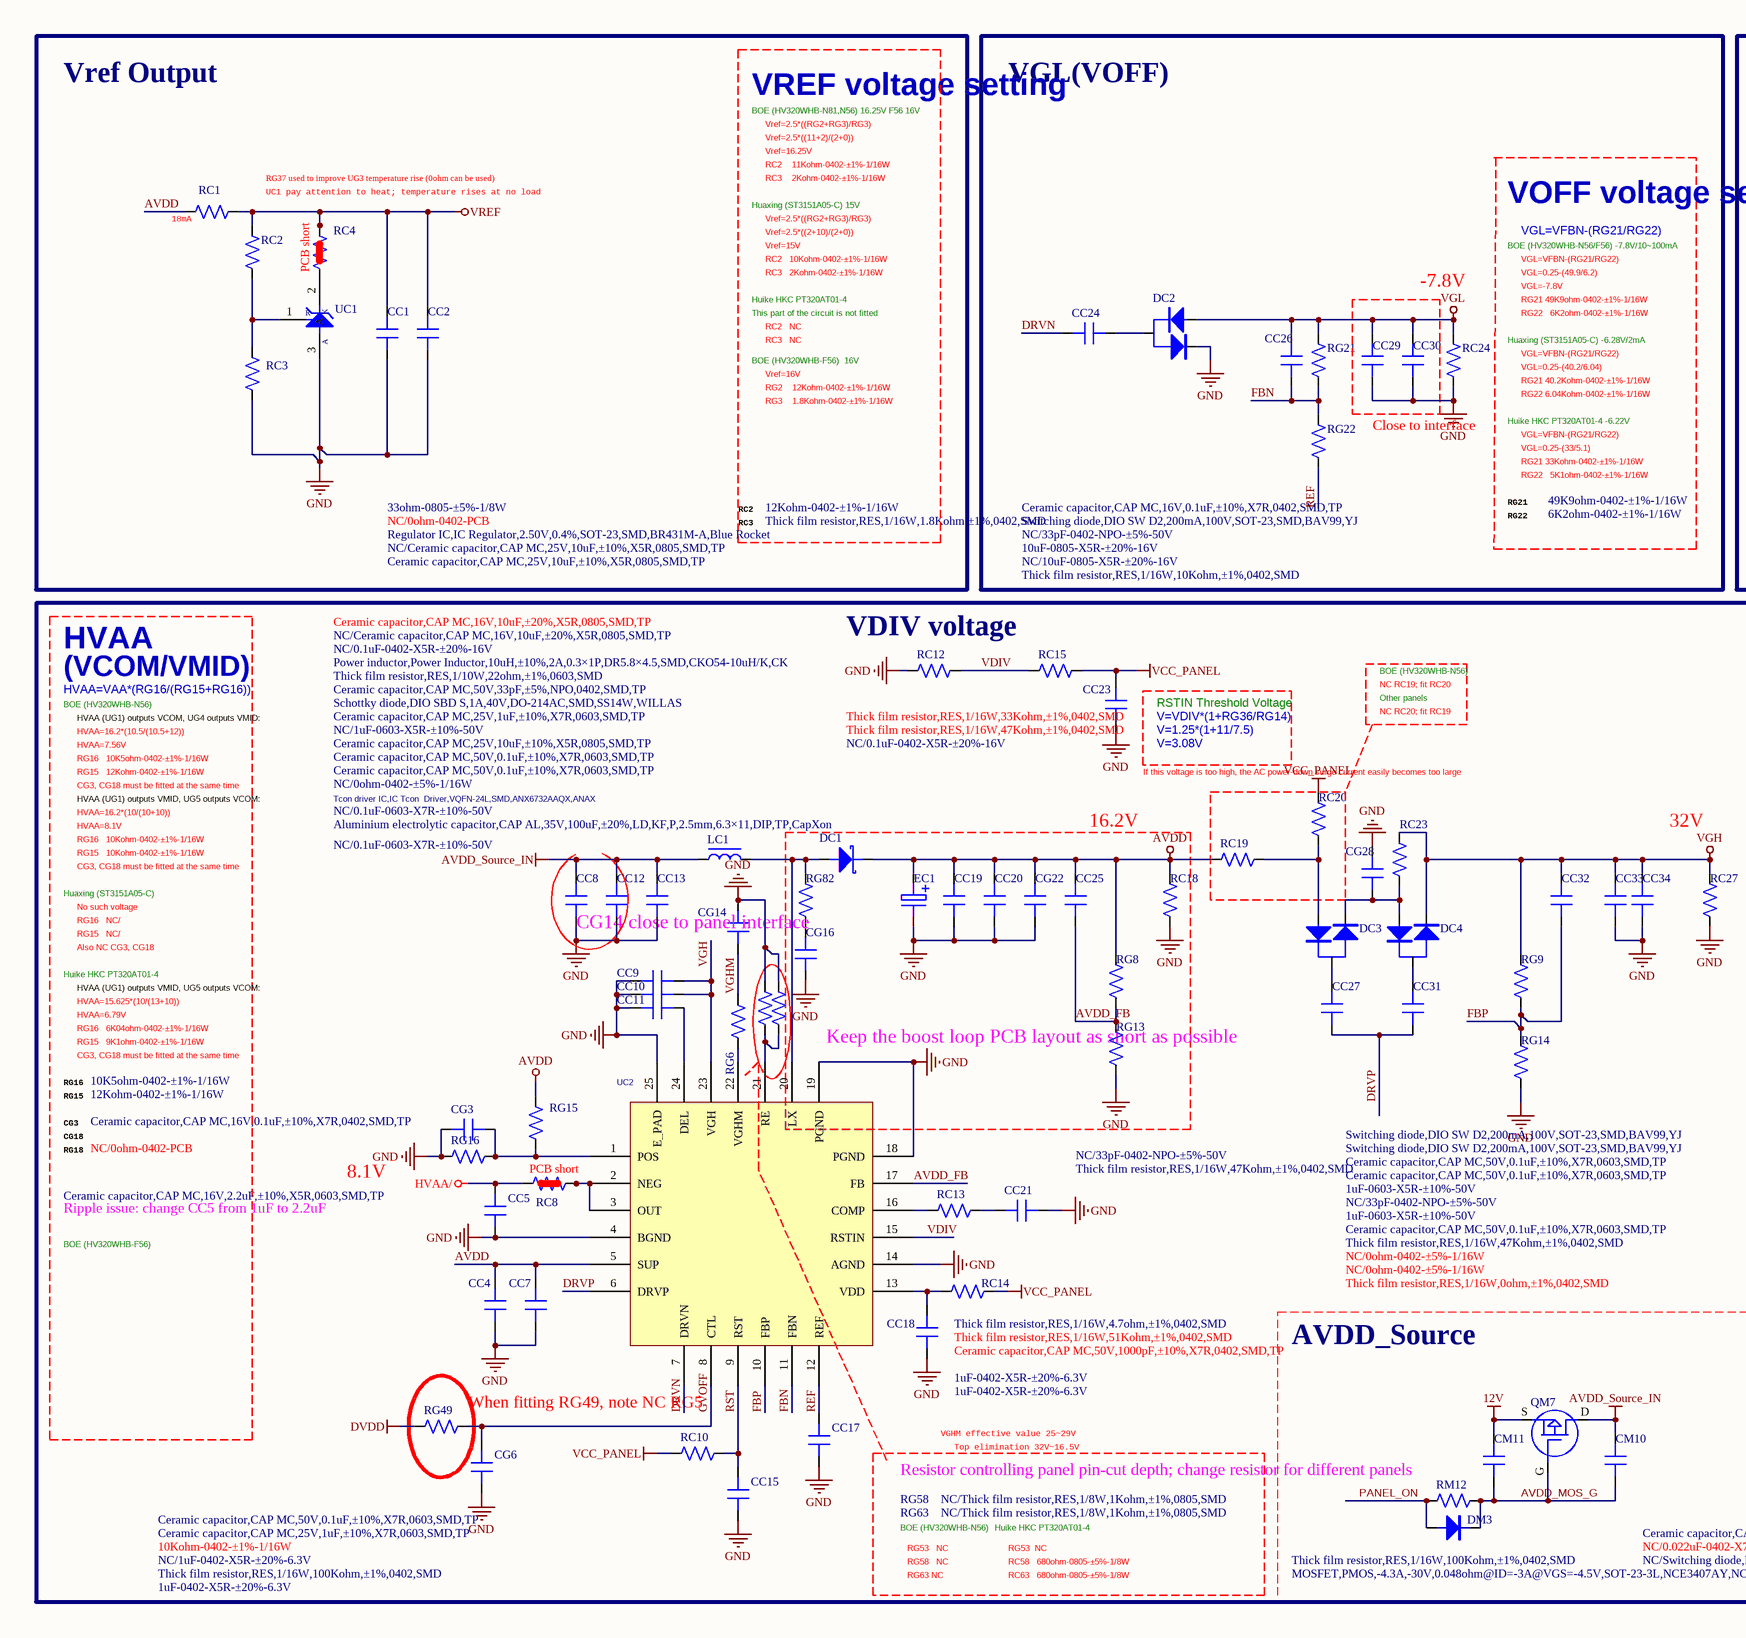
[diagram p0: MISC86383-19.SchDoc, left]
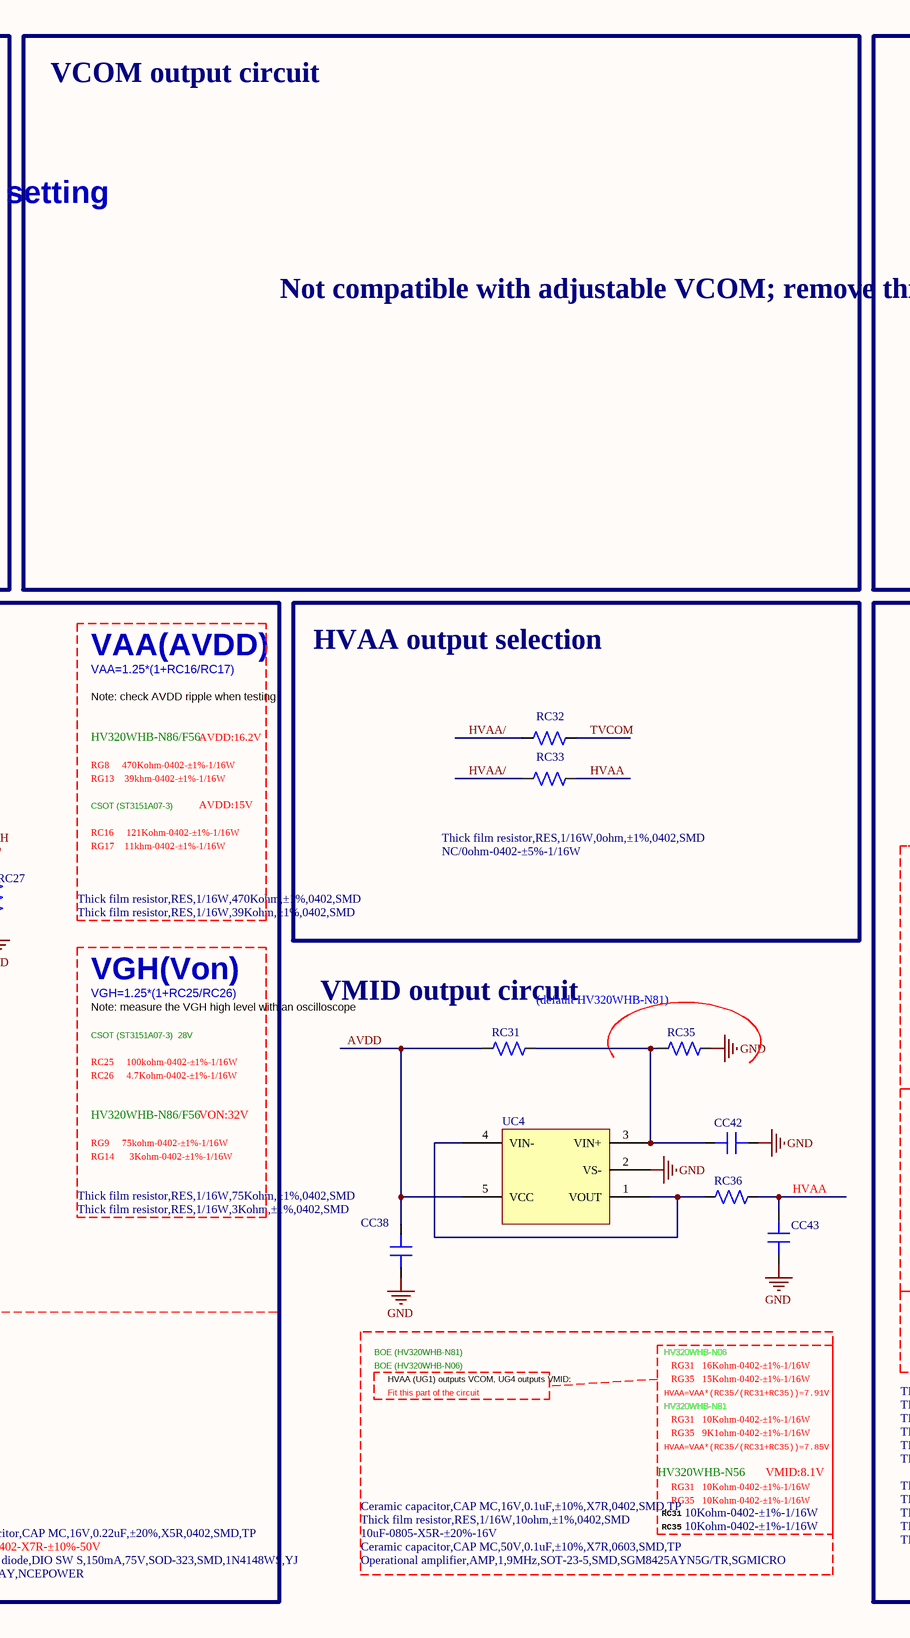
[diagram p1: MISC86383-19.SchDoc, middle]
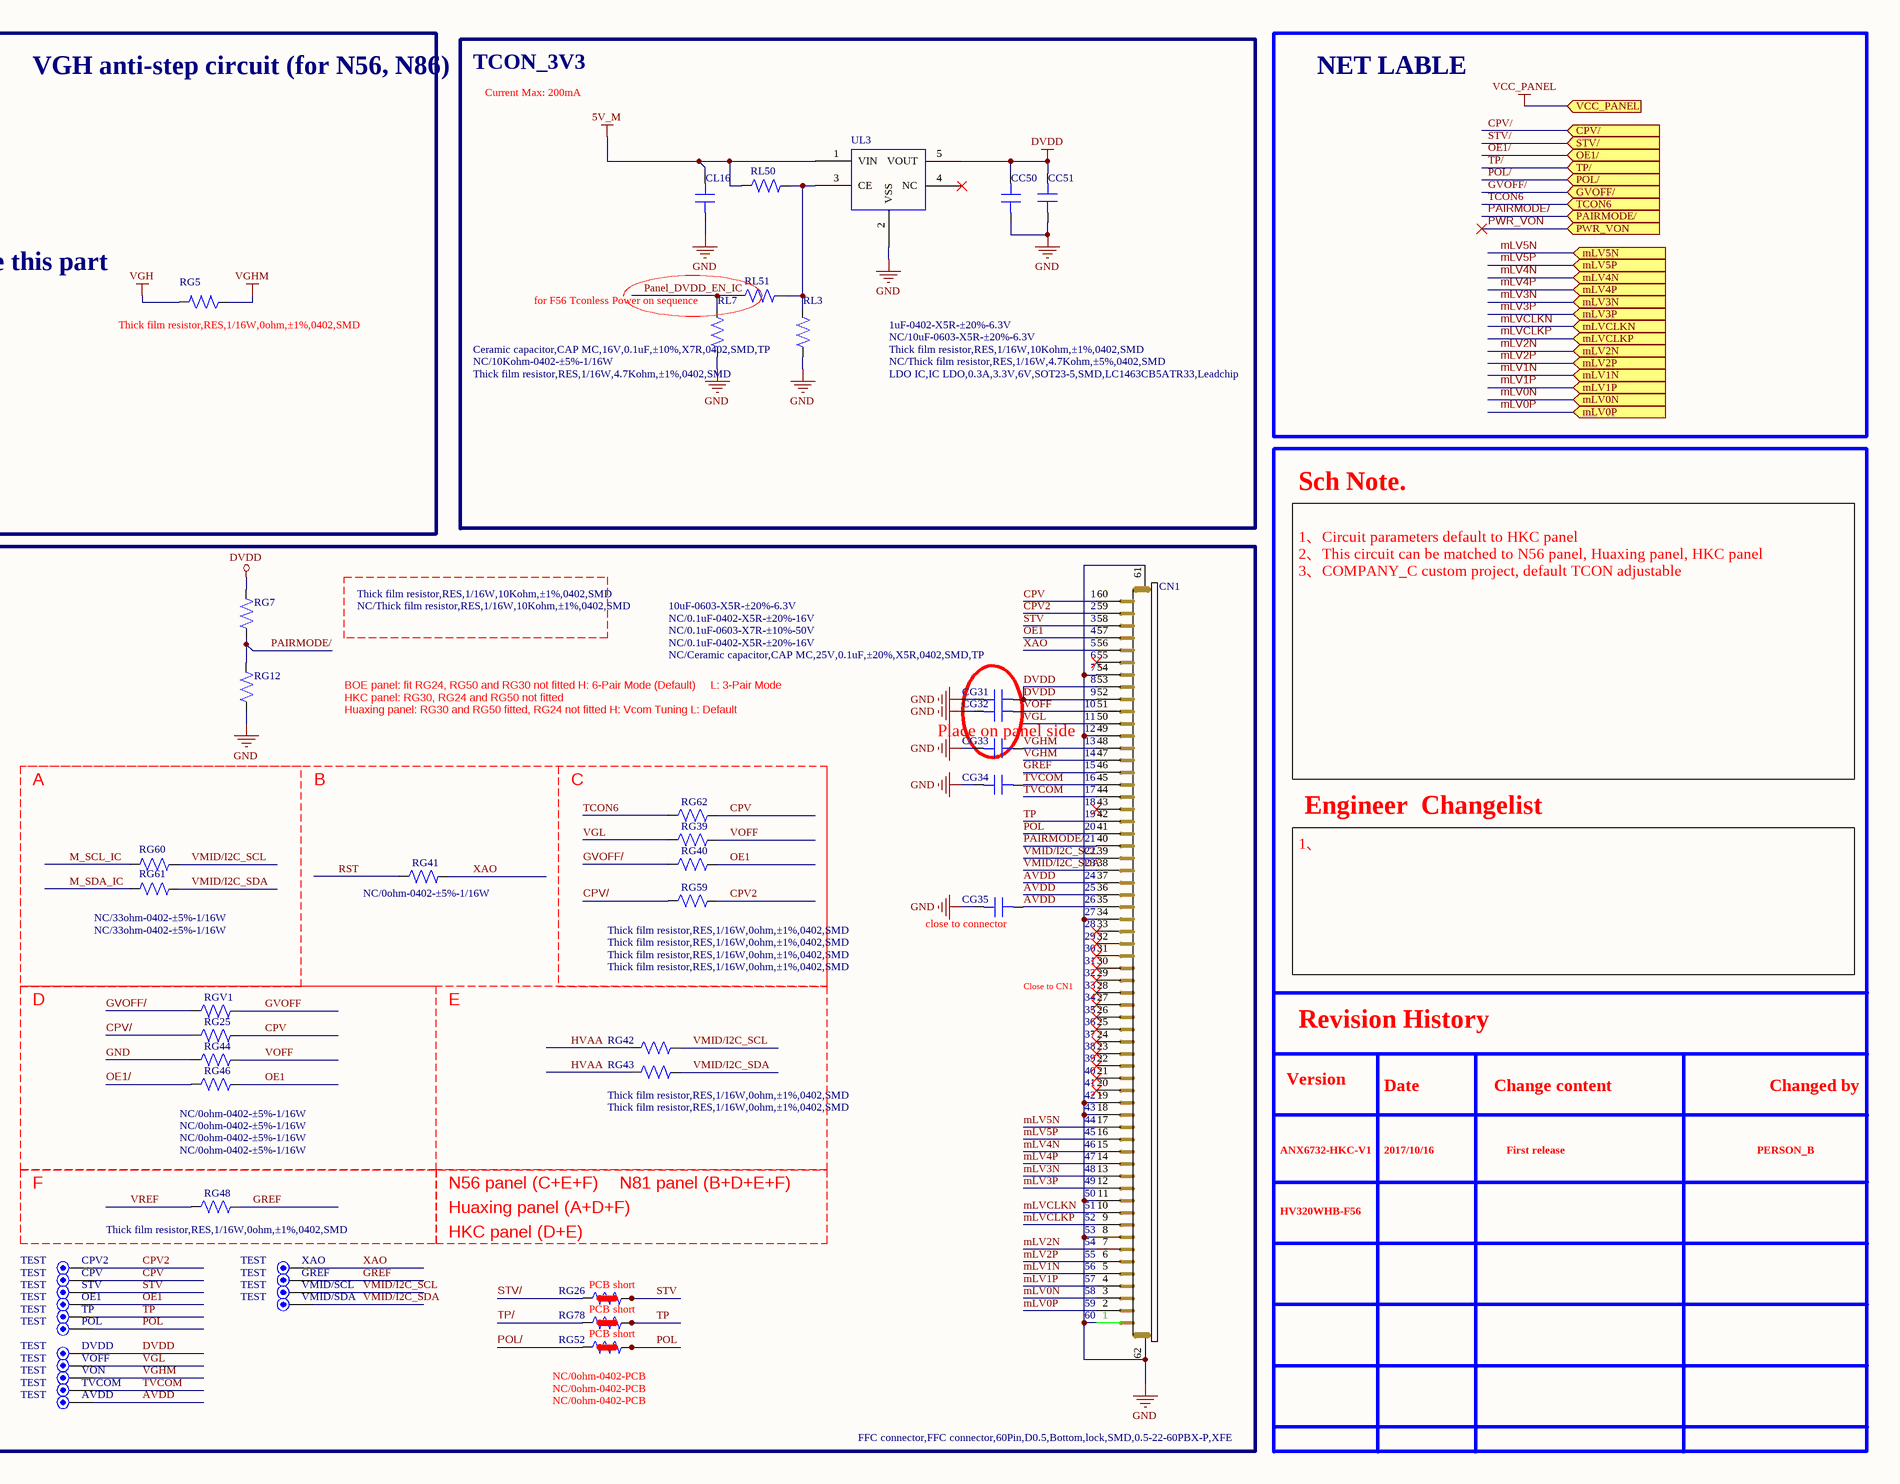
[diagram p2: MISC86383-19.SchDoc, right]
# Altium project MISC86383-33.PrjPCB (part 6 of 8)

## Sheet MISC86383-19.SchDoc
size 914 x 330 mm

### Parts
AVDD  TEST  [TP]
CC1  NC/Ceramic capacitor,CAP MC,25V,10uF,±10%,X5R,0805,SMD,TP  [C0805]
CC2  Ceramic capacitor,CAP MC,25V,10uF,±10%,X5R,0805,SMD,TP  [C0805]
CC4  Ceramic capacitor,CAP MC,25V,1uF,±10%,X7R,0603,SMD,TP  [C0603]
CC5  Ceramic capacitor,CAP MC,16V,2.2uF,±10%,X5R,0603,SMD,TP  [C0603]
CC7  Ceramic capacitor,CAP MC,50V,0.1uF,±10%,X7R,0603,SMD,TP  [C0603]
CC8  Ceramic capacitor,CAP MC,16V,10uF,±20%,X5R,0805,SMD,TP  [C0805]
CC9  NC/0.1uF-0603-X7R-±10%-50V  [C0603]
CC10  Ceramic capacitor,CAP MC,50V,0.1uF,±10%,X7R,0603,SMD,TP  [C0603]
CC11  Ceramic capacitor,CAP MC,50V,0.1uF,±10%,X7R,0603,SMD,TP  [C0603]
CC12  NC/Ceramic capacitor,CAP MC,16V,10uF,±20%,X5R,0805,SMD,TP  [C0805]
CC13  NC/0.1uF-0402-X5R-±20%-16V  [C0402]
CC15  1uF-0402-X5R-±20%-6.3V  [C0402]
CC17  1uF-0402-X5R-±20%-6.3V  [C0402]
CC18  1uF-0402-X5R-±20%-6.3V  [C0402]
CC19  Ceramic capacitor,CAP MC,25V,10uF,±10%,X5R,0805,SMD,TP  [C0805]
CC20  Ceramic capacitor,CAP MC,25V,1uF,±10%,X7R,0603,SMD,TP  [C0603]
CC21  Ceramic capacitor,CAP MC,50V,1000pF,±10%,X7R,0402,SMD,TP  [C0402]
CC23  NC/0.1uF-0402-X5R-±20%-16V  [C0402]
CC24  Ceramic capacitor,CAP MC,16V,0.1uF,±10%,X7R,0402,SMD,TP  [C0402]
CC25  NC/33pF-0402-NPO-±5%-50V  [C0402]
CC26  NC/33pF-0402-NPO-±5%-50V  [C0402]
CC27  Ceramic capacitor,CAP MC,50V,0.1uF,±10%,X7R,0603,SMD,TP  [C0603]
CC29  10uF-0805-X5R-±20%-16V  [C0805]
CC30  NC/10uF-0805-X5R-±20%-16V  [C0805]
CC31  Ceramic capacitor,CAP MC,50V,0.1uF,±10%,X7R,0603,SMD,TP  [C0603]
CC32  NC/33pF-0402-NPO-±5%-50V  [C0402]
CC33  1uF-0603-X5R-±10%-50V  [C0603]
CC34  Ceramic capacitor,CAP MC,50V,0.1uF,±10%,X7R,0603,SMD,TP  [C0603]
CC38  Ceramic capacitor,CAP MC,50V,0.1uF,±10%,X7R,0603,SMD,TP  [C0603]
CC42  Ceramic capacitor,CAP MC,16V,0.1uF,±10%,X7R,0402,SMD,TP  [C0402]
CC43  10uF-0805-X5R-±20%-16V  [C0805]
CC50  NC/10uF-0603-X5R-±20%-6.3V  [C0603]
CC51  1uF-0402-X5R-±20%-6.3V  [C0402]
CG3  Ceramic capacitor,CAP MC,16V,0.1uF,±10%,X7R,0402,SMD,TP  [C0402]
CG6  NC/1uF-0402-X5R-±20%-6.3V  [C0402]
CG14  NC/0.1uF-0603-X7R-±10%-50V  [C0603]
CG16  Ceramic capacitor,CAP MC,50V,33pF,±5%,NPO,0402,SMD,TP  [C0402]
CG22  NC/1uF-0603-X5R-±10%-50V  [C0603]
CG28  1uF-0603-X5R-±10%-50V  [C0603]
CG31  10uF-0603-X5R-±20%-6.3V  [C0603]
CG32  NC/0.1uF-0402-X5R-±20%-16V  [C0402]
CG33  NC/0.1uF-0603-X7R-±10%-50V  [C0603]
CG34  NC/0.1uF-0402-X5R-±20%-16V  [C0402]
CG35  NC/Ceramic capacitor,CAP MC,25V,0.1uF,±20%,X5R,0402,SMD,TP  [C0402]
CL16  Ceramic capacitor,CAP MC,16V,0.1uF,±10%,X7R,0402,SMD,TP  [C0402]
CM10  NC/0.022uF-0402-X7R-±10%-50V  [C0402]
CM11  Ceramic capacitor,CAP MC,16V,0.22uF,±20%,X5R,0402,SMD,TP  [C0402]
CN1  FFC connector,FFC connector,60Pin,D0.5,Bottom,lock,SMD,0.5-22-60PBX-P,XFE  [FFC60H/0.5S-11]
CPV  TEST  [TP]
CPV2  TEST  [TP]
DC1  Schottky diode,DIO SBD S,1A,40V,DO-214AC,SMD,SS14W,WILLAS  [DIODE-S-1]
DC2  Switching diode,DIO SW D2,200mA,100V,SOT-23,SMD,BAV99,YJ  [SO-23]
DC3  Switching diode,DIO SW D2,200mA,100V,SOT-23,SMD,BAV99,YJ  [SO-23]
DC4  Switching diode,DIO SW D2,200mA,100V,SOT-23,SMD,BAV99,YJ  [SO-23]
DM3  NC/Switching diode,DIO SW S,150mA,75V,SOD-323,SMD,1N4148WS,YJ  [DIODE-S-12]
DVDD  TEST  [TP]
EC1  Aluminium electrolytic capacitor,CAP AL,35V,100uF,±20%,LD,KF,P,2.5mm,6.3×11,DIP,TP,CapXon  [EC(6.3*11)-V-2.5]
GREF  TEST  [TP]
LC1  Power inductor,Power Inductor,10uH,±10%,2A,0.3×1P,DR5.8×4.5,SMD,CKO54-10uH/K,CK  [L(5.8*4.5)-S]
OE1  TEST  [TP]
POL  TEST  [TP]
QM7  MOSFET,PMOS,-4.3A,-30V,0.048ohm@ID=-3A@VGS=-4.5V,SOT-23-3L,NCE3407AY,NCEPOWER  [SOT-23-1]
RC1  33ohm-0805-±5%-1/8W  [R0805]
RC2  12Kohm-0402-±1%-1/16W  [R0402]
RC3  Thick film resistor,RES,1/16W,1.8Kohm,±1%,0402,SMD  [R0402]
RC4  NC/0ohm-0402-PCB  [R0402SC]
RC8  NC/0ohm-0402-PCB  [R0402SC]
RC10  Thick film resistor,RES,1/16W,100Kohm,±1%,0402,SMD  [R0402]
RC12  Thick film resistor,RES,1/16W,33Kohm,±1%,0402,SMD  [R0402]
RC13  Thick film resistor,RES,1/16W,51Kohm,±1%,0402,SMD  [R0402]
RC14  Thick film resistor,RES,1/16W,4.7ohm,±1%,0402,SMD  [R0402]
RC15  Thick film resistor,RES,1/16W,47Kohm,±1%,0402,SMD  [R0402]
RC18  Thick film resistor,RES,1/16W,47Kohm,±1%,0402,SMD  [R0402]
RC19  NC/0ohm-0402-±5%-1/16W  [R0402]
RC20  Thick film resistor,RES,1/16W,0ohm,±1%,0402,SMD  [R0402]
RC23  NC/0ohm-0402-±5%-1/16W  [R0402]
RC24  Thick film resistor,RES,1/16W,10Kohm,±1%,0402,SMD  [R0402]
RC27  Thick film resistor,RES,1/16W,47Kohm,±1%,0402,SMD  [R0402]
RC31  10Kohm-0402-±1%-1/16W  [R0402]
RC32  Thick film resistor,RES,1/16W,0ohm,±1%,0402,SMD  [R0402]
RC33  NC/0ohm-0402-±5%-1/16W  [R0402]
RC35  10Kohm-0402-±1%-1/16W  [R0402]
RC36  Thick film resistor,RES,1/16W,10ohm,±1%,0402,SMD  [R0402]
RG5  Thick film resistor,RES,1/16W,0ohm,±1%,0402,SMD  [R0402]
RG6  NC/0ohm-0402-±5%-1/16W  [R0402]
RG7  Thick film resistor,RES,1/16W,10Kohm,±1%,0402,SMD  [R0402]
RG8  Thick film resistor,RES,1/16W,470Kohm,±1%,0402,SMD  [R0402]
RG9  Thick film resistor,RES,1/16W,75Kohm,±1%,0402,SMD  [R0402]
RG12  NC/Thick film resistor,RES,1/16W,10Kohm,±1%,0402,SMD  [R0402]
RG13  Thick film resistor,RES,1/16W,39Kohm,±1%,0402,SMD  [R0402]
RG14  Thick film resistor,RES,1/16W,3Kohm,±1%,0402,SMD  [R0402]
RG15  12Kohm-0402-±1%-1/16W  [R0402]
RG16  10K5ohm-0402-±1%-1/16W  [R0402]
RG21  49K9ohm-0402-±1%-1/16W  [R0402]
RG22  6K2ohm-0402-±1%-1/16W  [R0402]
RG25  NC/0ohm-0402-±5%-1/16W  [R0402]
RG26  NC/0ohm-0402-PCB  [R0402SC]
RG39  Thick film resistor,RES,1/16W,0ohm,±1%,0402,SMD  [R0402]
RG40  Thick film resistor,RES,1/16W,0ohm,±1%,0402,SMD  [R0402]
RG41  NC/0ohm-0402-±5%-1/16W  [R0402]
RG42  Thick film resistor,RES,1/16W,0ohm,±1%,0402,SMD  [R0402]
RG43  Thick film resistor,RES,1/16W,0ohm,±1%,0402,SMD  [R0402]
RG44  NC/0ohm-0402-±5%-1/16W  [R0402]
RG46  NC/0ohm-0402-±5%-1/16W  [R0402]
RG48  Thick film resistor,RES,1/16W,0ohm,±1%,0402,SMD  [R0402]
RG49  10Kohm-0402-±1%-1/16W  [R0402]
RG52  NC/0ohm-0402-PCB  [R0402SC]
RG58  NC/Thick film resistor,RES,1/8W,1Kohm,±1%,0805,SMD  [R0805]
RG59  Thick film resistor,RES,1/16W,0ohm,±1%,0402,SMD  [R0402]
RG60  NC/33ohm-0402-±5%-1/16W  [R0402]
RG61  NC/33ohm-0402-±5%-1/16W  [R0402]
RG62  Thick film resistor,RES,1/16W,0ohm,±1%,0402,SMD  [R0402]
RG63  NC/Thick film resistor,RES,1/8W,1Kohm,±1%,0805,SMD  [R0805]
RG78  NC/0ohm-0402-PCB  [R0402SC]
RG82  Thick film resistor,RES,1/10W,22ohm,±1%,0603,SMD  [R0603]
RGV1  NC/0ohm-0402-±5%-1/16W  [R0402]
RL3  NC/Thick film resistor,RES,1/16W,4.7Kohm,±5%,0402,SMD  [R0402]
RL7  Thick film resistor,RES,1/16W,4.7Kohm,±1%,0402,SMD  [R0402]
RL50  NC/10Kohm-0402-±5%-1/16W  [R0402]
RL51  Thick film resistor,RES,1/16W,10Kohm,±1%,0402,SMD  [R0402]
RM12  Thick film resistor,RES,1/16W,100Kohm,±1%,0402,SMD  [R0402]
STV  TEST  [TP]
TP  TEST  [TP]
TVCOM  TEST  [TP]
UC1  Regulator IC,IC Regulator,2.50V,0.4%,SOT-23,SMD,BR431M-A,Blue Rocket  [SO-23-1]
UC2  Tcon driver IC,IC Tcon  Driver,VQFN-24L,SMD,ANX6732AAQX,ANAX  [QFN24/0.5-5]
UC4  Operational amplifier,AMP,1,9MHz,SOT-23-5,SMD,SGM8425AYN5G/TR,SGMICRO  [SOT-23-5]
UL3  LDO IC,IC LDO,0.3A,3.3V,6V,SOT23-5,SMD,LC1463CB5ATR33,Leadchip  [SOP23-5-1]
VMID/SCL  TEST  [TP]
VMID/SDA  TEST  [TP]
VOFF  TEST  [TP]
VON  TEST  [TP]
XAO  TEST  [TP]

### Blocks framed on the sheet
VREF voltage setting: CC1 CC2 RC1-RC4 UC1
VOFF voltage setting: CC24 CC26 DC2 RC24 RG21 RG22
VGH anti-step circuit (for N56, N86): RG5
TCON_3V3: CC50 CC51 CL16 RL3 RL7 RL50 RL51 UL3
-7.8V: CC29 CC30
HVAA output selection: RC32 RC33
A: RG60 RG61
C: RG39 RG40 RG59 RG62
F: RG48

### Ports
CPV/ (in), GVOFF/ (in), mLV0N (in), mLV0P (in), mLV1N (in), mLV1P (in), mLV2N (in), mLV2P (in), mLV3N (in), mLV3P (in), mLV4N (in), mLV4P (in), mLV5N (in), mLV5P (in), mLVCLKN (in), mLVCLKP (in), OE1/ (in), PAIRMODE/ (in), POL/ (in), PWR_VON (in), STV/ (in), TCON6 (in), TP/ (in), VCC_PANEL (in)

### Nets
5V_M: CL16.1 RL50.1 UL3.1(VIN)
12V: CM11.2 QM7.S
AVDD: AVDD.1 CC4.1 CC7.2 CC19.1 CC20.1 CC25.2 CC38.2 CG22.1 CG35.1 CN1.35 CN1.36 CN1.37 DC1.K EC1.1 RC1.1 RC18.2 RC19.2 RC31.1 RG8.2 RG15.2 UC2.5(SUP) UC4.5(VCC)
AVDD_Source_IN: CC8.2 CC12.2 CC13.2 CM10.1 LC1.1 QM7.D
DVDD: CC50.1 CC51.2 CG31.2 CN1.52 CN1.53 DVDD.1 RG7.2 RG49.2 UL3.5(VOUT)
GND: CC1.1 CC2.1 CC4.2 CC5.2 CC7.1 CC8.1 CC9.2 CC10.2 CC11.2 CC12.1 CC13.1 CC15.2 CC17.1 CC18.1 CC19.2 CC20.2 CC21.2 CC23.1 CC29.2 CC30.2 CC33.1 CC34.1 CC38.1 CC42.2 CC43.1 CC50.2 CC51.1 CG3.2 CG6.2 CG14.2 CG16.1 CG22.2 CG28.2 CG31.1 CG32.1 CG33.1 CG34.1 CG35.2 CL16.2 CN1.1 CN1.8 CN1.11 CN1.18 CN1.19 CN1.34 CN1.49 CN1.54 CN1.61 CN1.62 DC2.3 EC1.2 RC3.1 RC12.1 RC18.1 RC24.1 RC27.1 RC35.2 RG12.1 RG13.1 RG14.1 RG16.1 RG44.1 RG58.2 RG63.2 RL3.1 RL7.1 UC1.3(A) UC2.4(BGND) UC2.14(AGND) UC2.18(PGND) UC2.19(PGND) UC2.25(E_PAD) UC4.2(VS-) UL3.2(VSS)
HVAA/: CC5.1 RC8.1 RC32.2 RC33.1
VCC_PANEL: CC23.2 RC10.2 RC14.2 RC15.2 RC20.1 ; port VCC_PANEL
VGH: CC9.1 CC10.1 CC32.2 CC33.2 CC34.2 DC4.3 RC23.2 RC27.2 RG5.2 RG9.2 UC2.23(VGH)
VGHM: CG14.1 CG33.2 CN1.47 CN1.48 RG5.1 RG6.2 VON.1
VGL: CC26.2 CC29.1 CC30.1 CN1.50 DC2.1 RC24.2 RG21.2 RG39.1 VOFF.1
VREF: CC1.2 CC2.2 RC1.2 RC2.2 RC4.2 RC4.3 RG48.1
AVDD_FB: CC25.1 RG8.1 RG13.2 UC2.17(FB)
AVDD_MOS_G: CM10.2 CM11.1 DM3.K QM7.G RM12.2
CPV: CN1.60 CPV.1 RG25.2 RG62.2
CPV2: CN1.59 CPV2.1 RG59.2
CPV/: RG25.1 RG59.1 ; port CPV/
DRVN: CC24.1 UC2.7(DRVN)
DRVP: CC27.2 CC31.2 UC2.6(DRVP)
FBN: CC26.1 RG21.1 RG22.2 UC2.11(FBN)
FBP: CC32.1 RG9.1 RG14.2 UC2.10(FBP)
GREF: CN1.46 GREF.1 RG48.2
GVOFF: CG6.1 RG49.1 RGV1.2 UC2.8(CTL)
GVOFF/: RG40.1 RGV1.1 ; port GVOFF/
HVAA: CC43.2 RC33.2 RC36.2 RG42.1 RG43.1
M_SCL_IC: RG60.1
M_SDA_IC: RG61.1
mLV0N: CN1.3 ; port mLV0N
mLV0P: CN1.2 ; port mLV0P
mLV1N: CN1.5 ; port mLV1N
mLV1P: CN1.4 ; port mLV1P
mLV2N: CN1.7 ; port mLV2N
mLV2P: CN1.6 ; port mLV2P
mLV3N: CN1.13 ; port mLV3N
mLV3P: CN1.12 ; port mLV3P
mLV4N: CN1.15 ; port mLV4N
mLV4P: CN1.14 ; port mLV4P
mLV5N: CN1.17 ; port mLV5N
mLV5P: CN1.16 ; port mLV5P
mLVCLKN: CN1.10 ; port mLVCLKN
mLVCLKP: CN1.9 ; port mLVCLKP
OE1: CN1.57 OE1.1 RG40.2 RG46.2
OE1/: RG46.1 ; port OE1/
PAIRMODE/: CN1.40 RG7.1 RG12.2 ; port PAIRMODE/
Panel_DVDD_EN_IC: RL7.2 RL51.1
PANEL_ON: DM3.A RM12.1
POL: CN1.41 POL.1 RG52.2 RG52.3
POL/: RG52.1 ; port POL/
REF: CC17.2 RG22.1 UC2.12(REF)
RST: CC15.1 RC10.1 RG41.1 UC2.9(RST)
STV: CN1.58 RG26.2 RG26.3 STV.1
STV/: RG26.1 ; port STV/
TCON6: RG62.1 ; port TCON6
TP: CN1.42 RG78.2 RG78.3 TP.1
TP/: RG78.1 ; port TP/
TVCOM: CG34.2 CN1.44 CN1.45 RC32.1 TVCOM.1
VDIV: RC12.2 RC15.1 UC2.15(RSTIN)
VMID/I2C_SCL: CN1.39 RG42.2 RG60.2 VMID/SCL.1
VMID/I2C_SDA: CN1.38 RG43.2 RG61.2 VMID/SDA.1
VOFF: CG32.2 CN1.51 RG39.2 RG44.2
XAO: CN1.56 RG41.2 XAO.1
NetCC11_1: CC11.1 UC2.24(DEL)
NetCC18_2: CC18.2 RC14.1 UC2.13(VDD)
NetCC21_1: CC21.1 RC13.2
NetCC24_2: CC24.2 DC2.2
NetCC27_1: CC27.1 DC3.2
NetCC31_1: CC31.1 DC4.2
NetCC42_1: CC42.1 RC31.2 RC35.1 UC4.3(VIN+)
NetCG3_1: CG3.1 RG15.1 RG16.2 UC2.1(POS)
NetCG16_2: CG16.2 RG82.1
NetCG28_1: CG28.1 DC3.3 DC4.1 RC23.1
NetDC1_A: DC1.A LC1.2 RG82.2 UC2.20(LX)
NetDC3_1: DC3.1 RC19.1 RC20.2
NetRC2_1: RC2.1 RC3.2 UC1.1(R)
NetRC4_1: RC4.1 UC1.2(K)
NetRC8_2: RC8.2 RC8.3 UC2.2(NEG) UC2.3(OUT)
NetRC13_1: RC13.1 UC2.16(COMP)
NetRC36_1: RC36.1 UC4.1(VOUT) UC4.4(VIN-)
NetRG6_1: RG6.1 UC2.22(VGHM)
NetRG58_1: RG58.1 RG63.1 UC2.21(RE)
NetRL3_2: RL3.2 RL50.2 RL51.2 UL3.3(CE)

Not connected (* = marked no-connect by the designer): CN1 20* 21* 22* 23* 24* 25* 26* 27* 28* 29* 30* 31* 32* 33* 43* 55*; UL3 4(NC)*

### Notes on the sheet
- Vref Output
- VGL(VOFF)
- VCOM output circuit
- NET LABLE
- BOE (HV320WHB-N81,N56) 16.25V F56 16V
- Vref=2.5*((RG2+RG3)/RG3)
- Vref=2.5*((11+2)/(2+0))
- Vref=16.25V
- Current Max: 200mA
- (near RC1) 18mA
- UC1 pay attention to heat; temperature rises at no load
- RG37 used to improve UG3 temperature rise (0ohm can be used)
- Huaxing (ST3151A05-C) 15V
- RC2    11Kohm-0402-±1%-1/16W
- RC3    2Kohm-0402-±1%-1/16W
- Vref=2.5*((2+10)/(2+0))
- VGL=VFBN-(RG21/RG22)
- RC2   10Kohm-0402-±1%-1/16W
- RC3   2Kohm-0402-±1%-1/16W
- Vref=15V
- BOE (HV320WHB-N56/F56) -7.8V/10~100mA
- VGL=0.25-(49.9/6.2)
- VGL=-7.8V
- Huike HKC PT320AT01-4
- This part of the circuit is not fitted
- BOE (HV320WHB-F56)  16V
- RC2   NC
- RC3   NC
- Huaxing (ST3151A05-C) -6.28V/2mA
- VGL=0.25-(40.2/6.04)
- RG21 49K9ohm-0402-±1%-1/16W
- RG22   6K2ohm-0402-±1%-1/16W
- (near RG5) Not compatible with adjustable VCOM; remove this part
- (near RL7) for F56 Tconless Power on sequence
- RG2    12Kohm-0402-±1%-1/16W
- RG3    1.8Kohm-0402-±1%-1/16W
- Vref=16V
- Close to interface
- Huike HKC PT320AT01-4 -6.22V
- RG21 40.2Kohm-0402-±1%-1/16W
- RG22 6.04Kohm-0402-±1%-1/16W
- RG21
- VGL=0.25-(33/5.1)
- RG21 33Kohm-0402-±1%-1/16W
- RG22   5K1ohm-0402-±1%-1/16W
- RC3
- RC2
- RG22
- Sch Note.
- VDIV voltage
- HVAA
- (VCOM/VMID)
- HVAA=VAA*(RG16/(RG15+RG16))
- BOE (HV320WHB-N56)
- NC RC19; fit RC20
- Other panels
- VAA(AVDD)
- VAA=1.25*(1+RC16/RC17)
- Note: check AVDD ripple when testing
- (near CN1) 1
- (near CN1) 2
- (near CN1) 3
- (near CN1) 4
- RG16   10K5ohm-0402-±1%-1/16W
- HVAA=16.2*(10.5/(10.5+12))
- HVAA=7.56V
- HVAA (UG1) outputs VCOM, UG4 outputs VMID:
- RG15   12Kohm-0402-±1%-1/16W
- (near RC20) If this voltage is too high, the AC power-down surge current easily becomes too large
- (near CC23) V=VDIV*(1+RG36/RG14)
- (near CC23) V=1.25*(1+11/7.5)
- (near CC23) V=3.08V
- (near CC23) RSTIN Threshold Voltage
- NC RC20; fit RC19
- HV320WHB-N86/F56
- RG8     470Kohm-0402-±1%-1/16W
- AVDD:16.2V
- BOE panel: fit RG24, RG50 and RG30 not fitted H: 6-Pair Mode (Default)     L: 3-Pair Mode
- HKC panel: RG30, RG24 and RG50 not fitted
- (near CN1) 5
- (near CN1) 6
- (near CN1) 7
- (near CN1) 8
- (near CN1) 9
- HVAA=16.2*(10/(10+10))
- HVAA=8.1V
- CG3, CG18 must be fitted at the same time
- HVAA (UG1) outputs VMID, UG5 outputs VCOM:
- 16.2V
- 32V
- RG13    39khm-0402-±1%-1/16W
- RC16     121Kohm-0402-±1%-1/16W
- CSOT (ST3151A07-3)
- AVDD:15V
- Huaxing panel: RG30 and RG50 fitted, RG24 not fitted H: Vcom Tuning L: Default
- Place on panel side
- (near CN1) 10
- (near CN1) 11
- (near CN1) 12
- (near CN1) 13
- (near CN1) 14
- Huaxing (ST3151A05-C)
- RG16   10Kohm-0402-±1%-1/16W
- RG15   10Kohm-0402-±1%-1/16W
- No such voltage
- RG17    11khm-0402-±1%-1/16W
- B
- (near CN1) 15
- (near CN1) 16
- (near CN1) 17
- (near CN1) 18
- (near CN1) 19
- 1、Circuit parameters default to HKC panel
  2、This circuit can be matched to N56 panel, Huaxing panel, HKC panel
  3、COMPANY_C custom project, default TCON adjustable
- Engineer  Changelist
- RG16   NC/
- RG15   NC/
- Also NC CG3, CG18
- CG14 close to panel interface
- (near CN1) 20
- (near CN1) 21
- (near CN1) 22
- (near CN1) 23
- (near CN1) 24
- RG16   6K04ohm-0402-±1%-1/16W
- RG15   9K1ohm-0402-±1%-1/16W
- HVAA=15.625*(10/(13+10))
- HVAA=6.79V
- (near RG13) Keep the boost loop PCB layout as short as possible
- VGH(Von)
- Note: measure the VGH high level with an oscilloscope
- VGH=1.25*(1+RC25/RC26)
- CSOT (ST3151A07-3)  28V
- (near RC31) VMID output circuit
- (default HV320WHB-N81)
- (near CG35) close to connector
- (near CN1) 25
- (near CN1) 26
- (near CN1) 27
- (near CN1) 28
- (near CN1) 29
- RG16
- RG15
- RC25     100kohm-0402-±1%-1/16W
- RC26     4.7Kohm-0402-±1%-1/16W
- (near CN1) Close to CN1
- (near CN1) 30
- (near CN1) 31
- (near CN1) 32
- (near CN1) 33
- (near CN1) 34
- 1、
- RG18
- CG18
- CG3
- 8.1V
- RG9     75kohm-0402-±1%-1/16W
- RG14      3Kohm-0402-±1%-1/16W
- VON:32V
- D
- E
- (near CN1) 35
- (near CN1) 36
- (near CN1) 37
- (near CN1) 38
- (near CN1) 39
- Revision History
- Ripple issue: change CC5 from 1uF to 2.2uF
- (near CN1) 40
- (near CN1) 41
- (near CN1) 42
- (near CN1) 43
- (near CN1) 44
- Version
- Date
- Change content
- Changed by
- BOE (HV320WHB-F56)
- N56 panel (C+E+F)
- N81 panel (B+D+E+F)
- (near CN1) 45
- (near CN1) 46
- (near CN1) 47
- (near CN1) 48
- (near CN1) 49
- ANX6732-HKC-V1
- 2017/10/16
- First release
- PERSON_B
- AVDD_Source
- BOE (HV320WHB-N81)
- BOE (HV320WHB-N06)
- HV320WHB-N06
- RG31   16Kohm-0402-±1%-1/16W
- Huaxing panel (A+D+F)
- HKC panel (D+E)
- (near CN1) 50
- (near CN1) 51
- (near CN1) 52
- (near CN1) 53
- (near CN1) 54
- HV320WHB-F56
- (near RG49) When fitting RG49, note NC RG5
- VGHM effective value 25~29V
- Top elimination 32V~16.5V
- Fit this part of the circuit
- HVAA=VAA*(RC35/(RC31+RC35))=7.91V
- HV320WHB-N81
- HVAA=VAA*(RC35/(RC31+RC35))=7.85V
- RG35   15Kohm-0402-±1%-1/16W
- RG35   9K1ohm-0402-±1%-1/16W
- RG31   10Kohm-0402-±1%-1/16W
- (near CN1) 55
- (near CN1) 56
- (near CN1) 57
- (near CN1) 58
- (near CN1) 59
- Resistor controlling panel pin-cut depth; change resistor for different panels
- HV320WHB-N56
- RC31
- RG35   10Kohm-0402-±1%-1/16W
- VMID:8.1V
- (near CN1) 60
- RG53   NC
- RG58   NC
- RG63 NC
- RG53  NC
- RC58   680ohm-0805-±5%-1/8W
- RC63   680ohm-0805-±5%-1/8W
- RC35

### Library data of the parts
CC1 CC2 CC8 CC12 CC19 = 22uF-0805-X5R-±20%-6.3V-D
CC4 CC20 CC33 CG22 CG28 = 1uF-0603-X5R-±10%-50V-D
CC5 CC7 CC9-CC11 CC27 CC31 CC34 CC38 CG14 CG33 = 0.1uF-0603-X7R-±10%-50V-D: CAP
CC13 CG3 = 0.1uF-0402-Y5V-+80%-20%-16V-D
CC15 CC17 CC18 CG6 = 1uF-0402-X5R-±20%-16V-D
CC21 = 1500pF-0402-X7R-±10%-50V-D: CAP
CC23 CC24 CC42 CG32 CG34 CG35 CL16 = 0.1uF-0402-X5R-±20%-16V-D
CC25 CC26 CC32 = 33pF-0402-NPO-±5%-50V-D
CC29 CC30 CC43 = 10uF-0805-X5R-±20%-16V-D
CC50 CG31 = 10uF-0603-X5R-±20%-6.3V-D
CC51 = 1uF-0402-X5R-±20%-6.3V-D
CG16 = 68pF-0402-NPO-±5%-50V-D
CM10 = 0.022uF-0402-X7R-±10%-50V-D
CM11 = 004.003.0000398-D: Ceramic capacitor,CAP MC,16V,0.22uF,±20%,X5R,0402,SMD,TP-D
CN1 = XXX.XXX.0004396-D: FFC connector,FFC connector,60Pin,D0.5,Bottom,lock,SMD,0.5-22-60PBX-P,XFE-D
DC1 = SK34A-SMA-F-D
DC2-DC4 = BAT54S-D
DM3 = 1N4148WS-D
EC1 = 100uF-35V-±20%-6.3×11-105℃-KF-编带-F=2.5(CapXon)-DHAI: Electrolytic
LC1 = SCD54TL-6R8M-D
QM7 = 004.007.0000286-D: MOSFET,PMOS,-4.7A,-20V,70mohm@ID=-4.7A@VGS=-4.5V,SOT23-LC,LPB3443LT1G,LRC-D
RC1 = 10ohm-0805-±5%-1/8W-D
RC2 = 12Kohm-0402-±1%-1/16W-D
RC3 = 1K2ohm-0402-±1%-1/16W-D
RC4 RC8 RG26 RG52 RG78 = 0ohm-0402-PCB-D
RC10 RG49 = 100Kohm-0402-±5%-1/16W-D
RC12 = 56Kohm-0402-±1%-1/16W-D
RC13 RC18 RC27 = 47Kohm-0402-±5%-1/16W-D
RC14 = 4R7ohm-0402-±5%-1/16W-D
RC15 = 121Kohm-0402-±1%-1/16W-D
RC19 RC20 RC23 RC33 RG5 RG6 RG25 RG39-RG44 RG46 RG48 RG59 RG62 = 0ohm-0402-±5%-1/16W-D
RC24 RG7 RG12 RL50 RL51 = 10Kohm-0402-±5%-1/16W-D
RC31 RG16 = 16Kohm-0402-±1%-1/16W-D
RC32 = 10ohm-0402-±1%-1/16W-D
RC35 = 9K1ohm-0402-±1%-1/16W-D
RC36 RGV1 = 10ohm-0402-±5%-1/16W-D
RG8 = 470Kohm-0402-±1%-1/16W-D
RG9 = 100Kohm-0402-±1%-1/16W-D
RG13 = 39Kohm-0402-±1%-1/16W-D: RES
RG14 = 6K2ohm-0402-±1%-1/16W-D
RG15 = 18Kohm-0402-±1%-1/16W-D
RG21 = 62Kohm-0402-±1%-1/16W-D
RG22 = 7K5ohm-0402-±1%-1/16W-D
RG58 RG63 = 1Kohm-0805-±5%-1/8W-D
RG60 RG61 = 33ohm-0402-±5%-1/16W-D
RG82 = 10ohm-0603-±5%-1/10W-D
RL3 RL7 = 004.002.0000689-D: Thick film resistor,RES,1/16W,4.7Kohm,±5%,0402,SMD-D
RM12 = 004.002.0000578-D: Thick film resistor,RES,1/16W,100Kohm,±1%,0402,SMD-D
UC1 = TL431G-AE2-R(UTC)-D
UC2 = G5517-D
UC4 = 运算放大器,IC OP Amplifier,1 channel,18MHz,TSOT23-5,SMD,ANX7003AAK,ANAX
UL3 = 004.010.0000105-D: LDO IC,IC LDO,0.5A,3.3V,10V,SOT23-5,SMD,LC1458CB5TR33,LEADCHIP-D